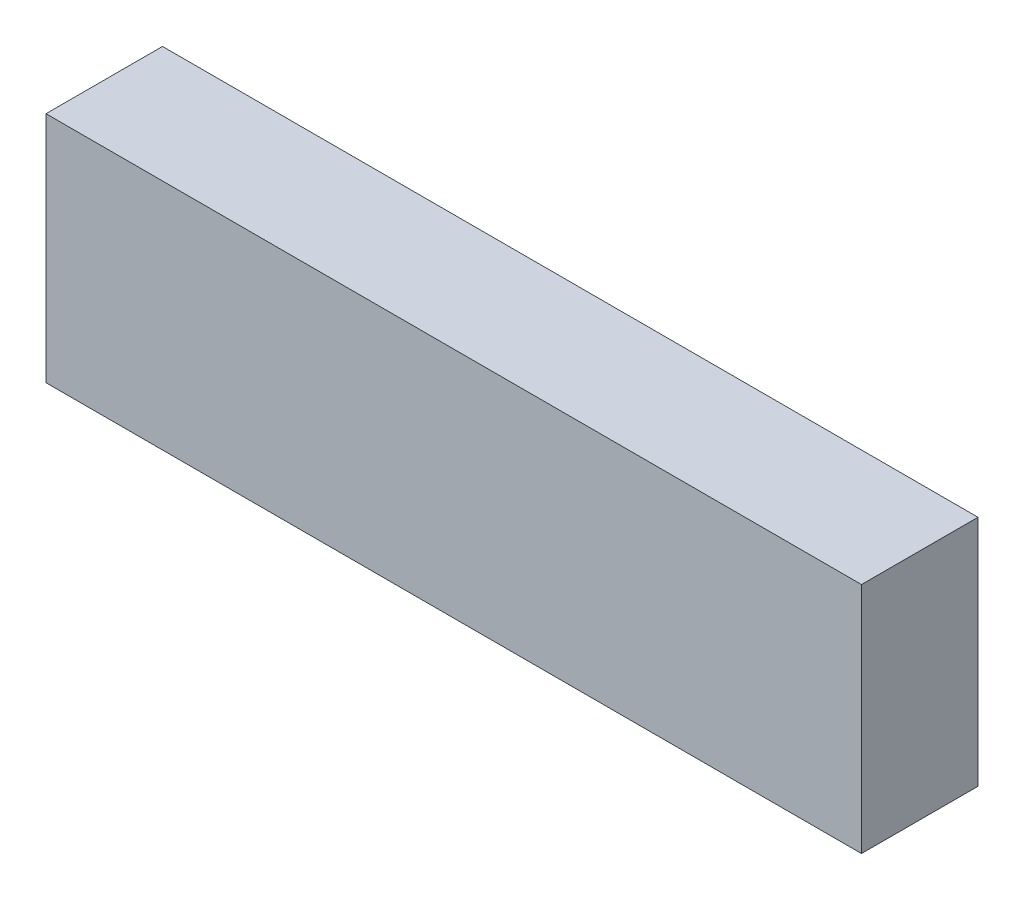
from build123d import *

# Parameters (mm, degrees)
SKETCH_1_W      = 70
SKETCH_1_H      = 20
EXTRUDE_1_DEPTH = 10


with BuildPart() as part:
    # 草图1 → 凸台-拉伸1 (new body)
    with BuildSketch(Plane.XY):
        Rectangle(SKETCH_1_W, SKETCH_1_H)
    extrude(amount=-EXTRUDE_1_DEPTH)


solid = part.part
